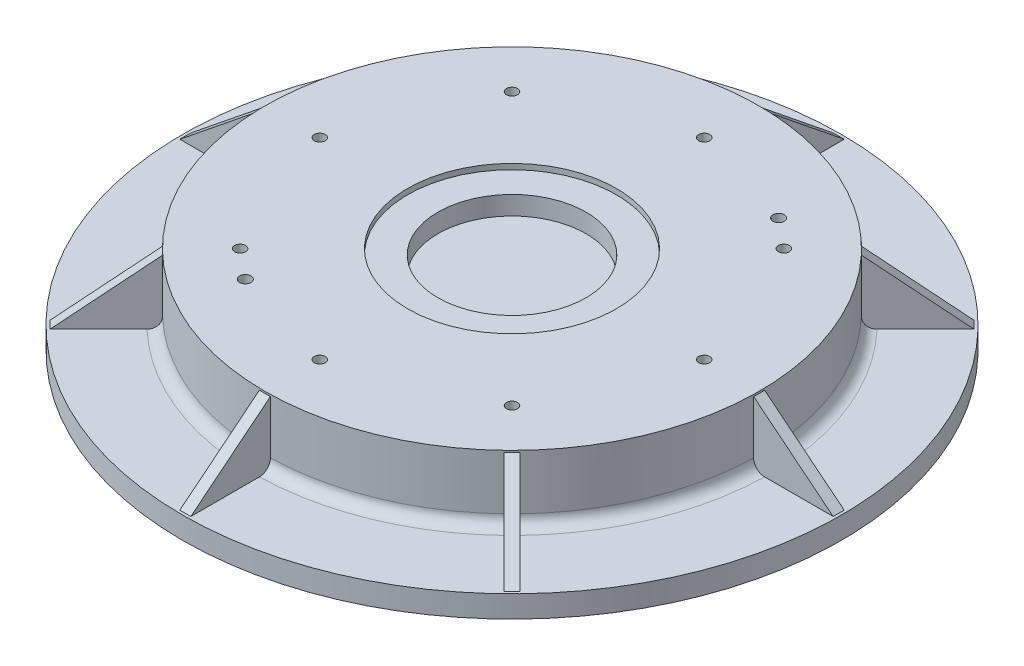
from build123d import *

# Parameters (mm, degrees)
RIB_2_REACH              = 429.222
SKETCH_2_WALL_W          = 949.398376266
SKETCH_2_WALL_H          = 10
PATTERN_CIRCULAR_1_COUNT = 8
SKETCH_4_R               = 13
CUT_EXTRUDE_1_DEPTH      = 2
CUT_EXTRUDE_2_REACH      = 430.77
SKETCH_5_R               = 6.5
CUT_EXTRUDE_3_REACH      = 437.89
SKETCH_6_R               = 5
SKETCH_6_R_2             = 15
SKETCH_7_R               = 4
CUT_EXTRUDE_5_DEPTH      = 67
SKETCH_8_R               = 13
EXTRUDE_1_DEPTH          = 20
SKETCH_9_R               = 15
EXTRUDE_2_DEPTH          = 20
EXTRUDE_START            = -52
SKETCH_10_R              = 7.5
EXTRUDE_3_DEPTH          = 52
SKETCH_12_R              = 205
SKETCH_12_R_2            = 65
SKETCH_12_R_3            = 5
EXTRUDE_4_DEPTH          = 10
SKETCH_16_R              = 67.5
CUT_EXTRUDE_6_DEPTH      = 22
SKETCH_17_R              = 95
CUT_EXTRUDE_7_DEPTH      = 5


with BuildPart() as part:
    # 草图1 → 旋转1 (revolve)
    with BuildSketch(Plane.XY, mode=Mode.PRIVATE) as revolve_1_sk:
        with BuildLine():
            Line((7.5, 50.18359375), (7.5, -1.81640625))
            Line((7.5, -1.81640625), (55, -1.81640625))
            Line((55, -1.81640625), (55, -41.81640625))
            Line((55, -41.81640625), (70, -41.81640625))
            Line((70, -41.81640625), (74.921875, 30.18359375))
            Line((74.921875, 30.18359375), (205, 30.18359375))
            Line((205, 30.18359375), (205, -49.81640625))
            Line((205, -49.81640625), (225, -49.81640625))
            Line((225, -49.81640625), (225, -29.81640625))
            Line((225, -29.81640625), (300, -29.81640625))
            Line((300, -29.81640625), (300, -9.81640625))
            Line((300, -9.81640625), (235, -9.81640625))
            ThreePointArc((235, -9.81640625), (227.928932188, -6.887474062), (225, 0.18359375))
            Line((225, 0.18359375), (225, 50.18359375))
            Line((225, 50.18359375), (7.5, 50.18359375))
        make_face()
    revolve(revolve_1_sk.sketch.rotate(Axis((0, 22.32421875, 0), (0, -1, 0)), 90), axis=Axis((0, 22.32421875, 0), (0, -1, 0)))

    # 草图2 wall → 筋2 (add, up to next)
    with BuildSketch(Plane(origin=(261.190811903, 19.344881739, 0), x_dir=(0.778674244513, -0.62742841897, 0), z_dir=(0.62742841897, 0.778674244513, 0)), mode=Mode.PRIVATE) as rib_2_sk1:
        Rectangle(SKETCH_2_WALL_W, SKETCH_2_WALL_H)
    rib_2_tool1 = extrude(rib_2_sk1.sketch, amount=-RIB_2_REACH, mode=Mode.PRIVATE) - part.part
    rib_2 = rib_2_tool1.solids().sort_by_distance((261.190811903, 19.344881739, 0))[0]
    add(rib_2)

    # 阵列(圆周)1: 筋2 ×8 about axis
    pattern_circular_1_axis = Axis((0, 0, 0), (0, 1, 0))
    for i in range(1, PATTERN_CIRCULAR_1_COUNT):
        add(rib_2.rotate(pattern_circular_1_axis, i * 360 / PATTERN_CIRCULAR_1_COUNT))

    # 草图4 → 切除-拉伸1 (cut)
    with BuildSketch(Plane(origin=(0, -9.81640625, 0), x_dir=(1, 0, 0), z_dir=(0, 1, 0))):
        with Locations(Location((235.58928079, -97.584275253, 0), (0, 0, 270))):
            Circle(SKETCH_4_R)
        with Locations(Location((97.584275253, -235.58928079, 0), (0, 0, 270))):
            Circle(SKETCH_4_R)
        with Locations(Location((-97.584275253, -235.58928079, 0), (0, 0, 270))):
            Circle(SKETCH_4_R)
        with Locations(Location((-235.58928079, -97.584275253, 0), (0, 0, 270))):
            Circle(SKETCH_4_R)
        with Locations(Location((-235.58928079, 97.584275253, 0), (0, 0, 270))):
            Circle(SKETCH_4_R)
        with Locations(Location((-97.584275253, 235.58928079, 0), (0, 0, 270))):
            Circle(SKETCH_4_R)
        with Locations(Location((97.584275253, 235.58928079, 0), (0, 0, 270))):
            Circle(SKETCH_4_R)
        with Locations(Location((235.58928079, 97.584275253, 0), (0, 0, 270))):
            Circle(SKETCH_4_R)
    extrude(amount=-CUT_EXTRUDE_1_DEPTH, mode=Mode.SUBTRACT)

    # 草图5 → 切除-拉伸2 (cut, up to next)
    with BuildSketch(Plane(origin=(0, -11.81640625, 0), x_dir=(1, 0, 0), z_dir=(0, 1, 0)), mode=Mode.PRIVATE) as cut_extrude_2_sk1:
        with Locations(Location((235.58928079, 97.584275253, 0), (0, 0, 270))):
            Circle(SKETCH_5_R)
    cut_extrude_2_tool1 = extrude(cut_extrude_2_sk1.sketch, amount=-CUT_EXTRUDE_2_REACH, mode=Mode.PRIVATE) & part.part
    # 草图5 → 切除-拉伸2 (cut, up to next)
    with BuildSketch(Plane(origin=(0, -11.81640625, 0), x_dir=(1, 0, 0), z_dir=(0, 1, 0)), mode=Mode.PRIVATE) as cut_extrude_2_sk2:
        with Locations(Location((235.58928079, -97.584275253, 0), (0, 0, 270))):
            Circle(SKETCH_5_R)
    cut_extrude_2_tool2 = extrude(cut_extrude_2_sk2.sketch, amount=-CUT_EXTRUDE_2_REACH, mode=Mode.PRIVATE) & part.part
    # 草图5 → 切除-拉伸2 (cut, up to next)
    with BuildSketch(Plane(origin=(0, -11.81640625, 0), x_dir=(1, 0, 0), z_dir=(0, 1, 0)), mode=Mode.PRIVATE) as cut_extrude_2_sk3:
        with Locations(Location((97.584275253, -235.58928079, 0), (0, 0, 270))):
            Circle(SKETCH_5_R)
    cut_extrude_2_tool3 = extrude(cut_extrude_2_sk3.sketch, amount=-CUT_EXTRUDE_2_REACH, mode=Mode.PRIVATE) & part.part
    # 草图5 → 切除-拉伸2 (cut, up to next)
    with BuildSketch(Plane(origin=(0, -11.81640625, 0), x_dir=(1, 0, 0), z_dir=(0, 1, 0)), mode=Mode.PRIVATE) as cut_extrude_2_sk4:
        with Locations(Location((-97.584275253, -235.58928079, 0), (0, 0, 270))):
            Circle(SKETCH_5_R)
    cut_extrude_2_tool4 = extrude(cut_extrude_2_sk4.sketch, amount=-CUT_EXTRUDE_2_REACH, mode=Mode.PRIVATE) & part.part
    # 草图5 → 切除-拉伸2 (cut, up to next)
    with BuildSketch(Plane(origin=(0, -11.81640625, 0), x_dir=(1, 0, 0), z_dir=(0, 1, 0)), mode=Mode.PRIVATE) as cut_extrude_2_sk5:
        with Locations(Location((-235.58928079, -97.584275253, 0), (0, 0, 270))):
            Circle(SKETCH_5_R)
    cut_extrude_2_tool5 = extrude(cut_extrude_2_sk5.sketch, amount=-CUT_EXTRUDE_2_REACH, mode=Mode.PRIVATE) & part.part
    # 草图5 → 切除-拉伸2 (cut, up to next)
    with BuildSketch(Plane(origin=(0, -11.81640625, 0), x_dir=(1, 0, 0), z_dir=(0, 1, 0)), mode=Mode.PRIVATE) as cut_extrude_2_sk6:
        with Locations(Location((-235.58928079, 97.584275253, 0), (0, 0, 270))):
            Circle(SKETCH_5_R)
    cut_extrude_2_tool6 = extrude(cut_extrude_2_sk6.sketch, amount=-CUT_EXTRUDE_2_REACH, mode=Mode.PRIVATE) & part.part
    # 草图5 → 切除-拉伸2 (cut, up to next)
    with BuildSketch(Plane(origin=(0, -11.81640625, 0), x_dir=(1, 0, 0), z_dir=(0, 1, 0)), mode=Mode.PRIVATE) as cut_extrude_2_sk7:
        with Locations(Location((-97.584275253, 235.58928079, 0), (0, 0, 270))):
            Circle(SKETCH_5_R)
    cut_extrude_2_tool7 = extrude(cut_extrude_2_sk7.sketch, amount=-CUT_EXTRUDE_2_REACH, mode=Mode.PRIVATE) & part.part
    # 草图5 → 切除-拉伸2 (cut, up to next)
    with BuildSketch(Plane(origin=(0, -11.81640625, 0), x_dir=(1, 0, 0), z_dir=(0, 1, 0)), mode=Mode.PRIVATE) as cut_extrude_2_sk8:
        with Locations(Location((97.584275253, 235.58928079, 0), (0, 0, 270))):
            Circle(SKETCH_5_R)
    cut_extrude_2_tool8 = extrude(cut_extrude_2_sk8.sketch, amount=-CUT_EXTRUDE_2_REACH, mode=Mode.PRIVATE) & part.part
    add(cut_extrude_2_tool1.solids().sort_by_distance((235.589281, -11.816406, -97.584275))[0], mode=Mode.SUBTRACT)
    add(cut_extrude_2_tool2.solids().sort_by_distance((235.589281, -11.816406, 97.584275))[0], mode=Mode.SUBTRACT)
    add(cut_extrude_2_tool3.solids().sort_by_distance((97.584275, -11.816406, 235.589281))[0], mode=Mode.SUBTRACT)
    add(cut_extrude_2_tool4.solids().sort_by_distance((-97.584275, -11.816406, 235.589281))[0], mode=Mode.SUBTRACT)
    add(cut_extrude_2_tool5.solids().sort_by_distance((-235.589281, -11.816406, 97.584275))[0], mode=Mode.SUBTRACT)
    add(cut_extrude_2_tool6.solids().sort_by_distance((-235.589281, -11.816406, -97.584275))[0], mode=Mode.SUBTRACT)
    add(cut_extrude_2_tool7.solids().sort_by_distance((-97.584275, -11.816406, -235.589281))[0], mode=Mode.SUBTRACT)
    add(cut_extrude_2_tool8.solids().sort_by_distance((97.584275, -11.816406, -235.589281))[0], mode=Mode.SUBTRACT)

    # 草图6 → 切除-拉伸3 (cut, up to next)
    with BuildSketch(Plane(origin=(0, 50.18359375, 0), x_dir=(1, 0, 0), z_dir=(0, 1, 0)), mode=Mode.PRIVATE) as cut_extrude_3_sk1:
        with Locations(Location((175, 0, 0), (0, 0, 270))):
            Circle(SKETCH_6_R)
    cut_extrude_3_tool1 = extrude(cut_extrude_3_sk1.sketch, amount=-CUT_EXTRUDE_3_REACH, mode=Mode.PRIVATE) & part.part
    # 草图6 → 切除-拉伸3 (cut, up to next)
    with BuildSketch(Plane(origin=(0, 50.18359375, 0), x_dir=(1, 0, 0), z_dir=(0, 1, 0)), mode=Mode.PRIVATE) as cut_extrude_3_sk2:
        with Locations(Location((123.743686708, -123.743686708, 0), (0, 0, 270))):
            Circle(SKETCH_6_R)
    cut_extrude_3_tool2 = extrude(cut_extrude_3_sk2.sketch, amount=-CUT_EXTRUDE_3_REACH, mode=Mode.PRIVATE) & part.part
    # 草图6 → 切除-拉伸3 (cut, up to next)
    with BuildSketch(Plane(origin=(0, 50.18359375, 0), x_dir=(1, 0, 0), z_dir=(0, 1, 0)), mode=Mode.PRIVATE) as cut_extrude_3_sk3:
        with Locations(Location((0, -175, 0), (0, 0, 270))):
            Circle(SKETCH_6_R)
    cut_extrude_3_tool3 = extrude(cut_extrude_3_sk3.sketch, amount=-CUT_EXTRUDE_3_REACH, mode=Mode.PRIVATE) & part.part
    # 草图6 → 切除-拉伸3 (cut, up to next)
    with BuildSketch(Plane(origin=(0, 50.18359375, 0), x_dir=(1, 0, 0), z_dir=(0, 1, 0)), mode=Mode.PRIVATE) as cut_extrude_3_sk4:
        with Locations(Location((-123.743686708, -123.743686708, 0), (0, 0, 270))):
            Circle(SKETCH_6_R)
    cut_extrude_3_tool4 = extrude(cut_extrude_3_sk4.sketch, amount=-CUT_EXTRUDE_3_REACH, mode=Mode.PRIVATE) & part.part
    # 草图6 → 切除-拉伸3 (cut, up to next)
    with BuildSketch(Plane(origin=(0, 50.18359375, 0), x_dir=(1, 0, 0), z_dir=(0, 1, 0)), mode=Mode.PRIVATE) as cut_extrude_3_sk5:
        with Locations(Location((-175, 0, 0), (0, 0, 270))):
            Circle(SKETCH_6_R)
    cut_extrude_3_tool5 = extrude(cut_extrude_3_sk5.sketch, amount=-CUT_EXTRUDE_3_REACH, mode=Mode.PRIVATE) & part.part
    # 草图6 → 切除-拉伸3 (cut, up to next)
    with BuildSketch(Plane(origin=(0, 50.18359375, 0), x_dir=(1, 0, 0), z_dir=(0, 1, 0)), mode=Mode.PRIVATE) as cut_extrude_3_sk6:
        with Locations(Location((-123.743686708, 123.743686708, 0), (0, 0, 270))):
            Circle(SKETCH_6_R)
    cut_extrude_3_tool6 = extrude(cut_extrude_3_sk6.sketch, amount=-CUT_EXTRUDE_3_REACH, mode=Mode.PRIVATE) & part.part
    # 草图6 → 切除-拉伸3 (cut, up to next)
    with BuildSketch(Plane(origin=(0, 50.18359375, 0), x_dir=(1, 0, 0), z_dir=(0, 1, 0)), mode=Mode.PRIVATE) as cut_extrude_3_sk7:
        with Locations(Location((0, 175, 0), (0, 0, 270))):
            Circle(SKETCH_6_R)
    cut_extrude_3_tool7 = extrude(cut_extrude_3_sk7.sketch, amount=-CUT_EXTRUDE_3_REACH, mode=Mode.PRIVATE) & part.part
    # 草图6 → 切除-拉伸3 (cut, up to next)
    with BuildSketch(Plane(origin=(0, 50.18359375, 0), x_dir=(1, 0, 0), z_dir=(0, 1, 0)), mode=Mode.PRIVATE) as cut_extrude_3_sk8:
        with Locations(Location((123.743686708, 123.743686708, 0), (0, 0, 270))):
            Circle(SKETCH_6_R)
    cut_extrude_3_tool8 = extrude(cut_extrude_3_sk8.sketch, amount=-CUT_EXTRUDE_3_REACH, mode=Mode.PRIVATE) & part.part
    # 草图6 → 切除-拉伸3 (cut, up to next)
    with BuildSketch(Plane(origin=(0, 50.18359375, 0), x_dir=(1, 0, 0), z_dir=(0, 1, 0)), mode=Mode.PRIVATE) as cut_extrude_3_sk9:
        with Locations(Location((-125, 74, 0), (0, 0, 270))):
            Circle(SKETCH_6_R_2)
    cut_extrude_3_tool9 = extrude(cut_extrude_3_sk9.sketch, amount=-CUT_EXTRUDE_3_REACH, mode=Mode.PRIVATE) & part.part
    add(cut_extrude_3_tool1.solids().sort_by_distance((175, 50.183594, 0))[0], mode=Mode.SUBTRACT)
    add(cut_extrude_3_tool2.solids().sort_by_distance((123.743687, 50.183594, 123.743687))[0], mode=Mode.SUBTRACT)
    add(cut_extrude_3_tool3.solids().sort_by_distance((0, 50.183594, 175))[0], mode=Mode.SUBTRACT)
    add(cut_extrude_3_tool4.solids().sort_by_distance((-123.743687, 50.183594, 123.743687))[0], mode=Mode.SUBTRACT)
    add(cut_extrude_3_tool5.solids().sort_by_distance((-175, 50.183594, 0))[0], mode=Mode.SUBTRACT)
    add(cut_extrude_3_tool6.solids().sort_by_distance((-123.743687, 50.183594, -123.743687))[0], mode=Mode.SUBTRACT)
    add(cut_extrude_3_tool7.solids().sort_by_distance((0, 50.183594, -175))[0], mode=Mode.SUBTRACT)
    add(cut_extrude_3_tool8.solids().sort_by_distance((123.743687, 50.183594, -123.743687))[0], mode=Mode.SUBTRACT)
    add(cut_extrude_3_tool9.solids().sort_by_distance((-125, 50.183594, -74))[0], mode=Mode.SUBTRACT)

    # 草图7 → 切除-拉伸5 (cut)
    with BuildSketch(Plane.XZ.offset(41.81640625)):
        with Locations(Location((0, 43, 0), (0, 0, 270))):
            Circle(SKETCH_7_R)
        with Locations(Location((30.405591591, 30.405591591, 0), (0, 0, 270))):
            Circle(SKETCH_7_R)
        with Locations(Location((43, 0, 0), (0, 0, 270))):
            Circle(SKETCH_7_R)
        with Locations(Location((30.405591591, -30.405591591, 0), (0, 0, 270))):
            Circle(SKETCH_7_R)
        with Locations(Location((0, -43, 0), (0, 0, 270))):
            Circle(SKETCH_7_R)
        with Locations(Location((-30.405591591, -30.405591591, 0), (0, 0, 270))):
            Circle(SKETCH_7_R)
        with Locations(Location((-43, 0, 0), (0, 0, 270))):
            Circle(SKETCH_7_R)
        with Locations(Location((-30.405591591, 30.405591591, 0), (0, 0, 270))):
            Circle(SKETCH_7_R)
    extrude(amount=-CUT_EXTRUDE_5_DEPTH, mode=Mode.SUBTRACT)

    # 草图8 → 凸台-拉伸1 (add)
    with BuildSketch(Plane(origin=(0, -9.81640625, 0), x_dir=(1, 0, 0), z_dir=(0, 1, 0))):
        with Locations((-235.58928079, 97.584275253)):
            Circle(SKETCH_8_R)
        with Locations((-235.58928079, -97.584275253)):
            Circle(SKETCH_8_R)
        with Locations((-97.584275253, -235.58928079)):
            Circle(SKETCH_8_R)
        with Locations((97.584275253, -235.58928079)):
            Circle(SKETCH_8_R)
        with Locations((235.58928079, -97.584275253)):
            Circle(SKETCH_8_R)
        with Locations((235.58928079, 97.584275253)):
            Circle(SKETCH_8_R)
        with Locations((97.584275253, 235.58928079)):
            Circle(SKETCH_8_R)
        with Locations((-97.584275253, 235.58928079)):
            Circle(SKETCH_8_R)
    extrude(amount=-EXTRUDE_1_DEPTH)

    # 草图9 → 凸台-拉伸2 (add)
    with BuildSketch(Plane(origin=(0, 50.18359375, 0), x_dir=(1, 0, 0), z_dir=(0, 1, 0))):
        with Locations((-125, 74)):
            Circle(SKETCH_9_R)
    extrude(amount=-EXTRUDE_2_DEPTH)

    # 草图10 → 凸台-拉伸3 (add)
    with BuildSketch(Plane(origin=(0, 50.18359375, 0), x_dir=(1, 0, 0), z_dir=(0, 1, 0)).offset(EXTRUDE_START)):
        Circle(SKETCH_10_R)
    extrude(amount=EXTRUDE_3_DEPTH)

    # 草图12 → 凸台-拉伸4 (add)
    with BuildSketch(Plane.XZ.offset(-30.18359375)):
        with Locations(Location((0, 0, 0), (0, 0, 90))):
            Circle(SKETCH_12_R)
        Circle(SKETCH_12_R_2, mode=Mode.SUBTRACT)
        with Locations(Location((123.743686708, -123.743686708, 0), (0, 0, 90))):
            Circle(SKETCH_12_R_3, mode=Mode.SUBTRACT)
        with Locations(Location((0, -175, 0), (0, 0, 90))):
            Circle(SKETCH_12_R_3, mode=Mode.SUBTRACT)
        with Locations(Location((-123.743686708, -123.743686708, 0), (0, 0, 90))):
            Circle(SKETCH_12_R_3, mode=Mode.SUBTRACT)
        with Locations(Location((-175, 0, 0), (0, 0, 90))):
            Circle(SKETCH_12_R_3, mode=Mode.SUBTRACT)
        with Locations(Location((175, 0, 0), (0, 0, 90))):
            Circle(SKETCH_12_R_3, mode=Mode.SUBTRACT)
        with Locations(Location((123.743686708, 123.743686708, 0), (0, 0, 90))):
            Circle(SKETCH_12_R_3, mode=Mode.SUBTRACT)
        with Locations(Location((-123.743686708, 123.743686708, 0), (0, 0, 90))):
            Circle(SKETCH_12_R_3, mode=Mode.SUBTRACT)
        with Locations(Location((0, 175, 0), (0, 0, 90))):
            Circle(SKETCH_12_R_3, mode=Mode.SUBTRACT)
    extrude(amount=EXTRUDE_4_DEPTH)

    # 草图16 → 切除-拉伸6 (cut)
    with BuildSketch(Plane(origin=(0, 50.18359375, 0), x_dir=(1, 0, 0), z_dir=(0, 1, 0))):
        with Locations(Location((0, 0, 0), (0, 0, 270))):
            Circle(SKETCH_16_R)
    extrude(amount=-CUT_EXTRUDE_6_DEPTH, mode=Mode.SUBTRACT)

    # 草图17 → 切除-拉伸7 (cut)
    with BuildSketch(Plane(origin=(0, 50.18359375, 0), x_dir=(1, 0, 0), z_dir=(0, 1, 0))):
        with Locations(Location((0, 0, 0), (0, 0, 270))):
            Circle(SKETCH_17_R)
    extrude(amount=-CUT_EXTRUDE_7_DEPTH, mode=Mode.SUBTRACT)

    # 草图20 → 切除-旋转1 (revolve, cut)
    with BuildSketch(Plane(origin=(0, 62.303737558, 0), x_dir=(0, -1, 0), z_dir=(0.8314696123025378, 0, 0.5555702330196134)), mode=Mode.PRIVATE) as cut_revolve_1_sk:
        Polygon((22.120143808, 175), (-27.879856192, 175), (-27.879856192, 181), (22.120143808, 180), align=None)
    cut_revolve_1 = revolve(cut_revolve_1_sk.sketch.rotate(Axis((97.224790778, 40.18359375, -145.507182153), (0, 1, 0)), 213.75), axis=Axis((97.224790778, 40.18359375, -145.507182153), (0, 1, 0)), mode=Mode.SUBTRACT)

    # 镜向1: 切除-旋转1 across plane
    add(cut_revolve_1.mirror(Plane(origin=(0, 0, 0), x_dir=(0.831469612302494, 0, 0.555570233019679), z_dir=(-0.5555702330196793, 0, 0.8314696123024938))), mode=Mode.SUBTRACT)


solid = part.part
